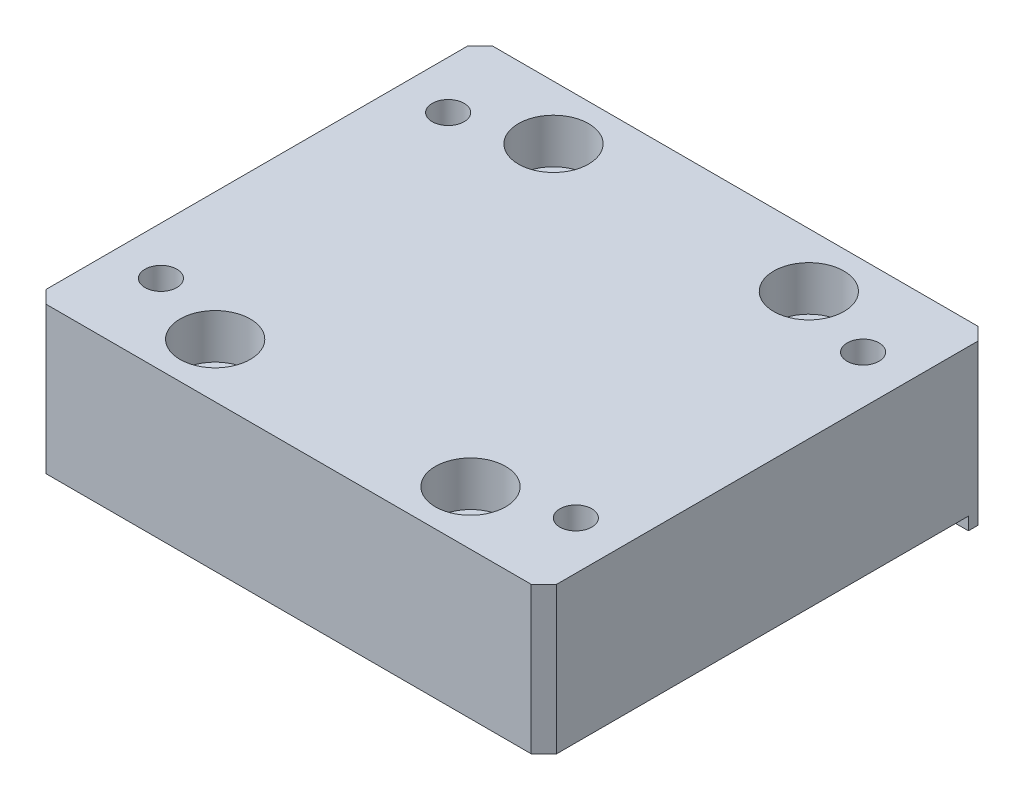
from build123d import *

# Parameters (mm, degrees)
SKETCH_1_W                = 80
SKETCH_1_H                = 70
EXTRUDE_1_DEPTH           = 12.5
SKETCH_3_W                = 80
SKETCH_3_H                = 66.5
CUT_EXTRUDE_1_DEPTH       = 2
HOLE_WIZARD_M5_1_D        = 4.2
HOLE_WIZARD_M6_1_D        = 5
CHAMFER_1_SIZE            = 2
HOLE_WIZARD_1_D           = 6.6
HOLE_WIZARD_1_DEPTH       = 25
HOLE_WIZARD_1_CBORE_D     = 11
HOLE_WIZARD_1_CBORE_DEPTH = 7


with BuildPart() as part:
    # 草图1 → 凸台-拉伸1 (new, symmetric)
    with BuildSketch(Plane(origin=(0, 0, 0), x_dir=(1, 0, 0), z_dir=(0, 1, 0))):
        Rectangle(SKETCH_1_W, SKETCH_1_H)
    extrude(amount=EXTRUDE_1_DEPTH, both=True)

    # 草图3 → 切除-拉伸1 (cut)
    with BuildSketch(Plane.XZ.offset(12.5)):
        with Locations((0, 1.75)):
            Rectangle(SKETCH_3_W, SKETCH_3_H)
    extrude(amount=-CUT_EXTRUDE_1_DEPTH, mode=Mode.SUBTRACT)

    # M5 螺纹孔1 (through all)
    with Locations(Plane(origin=(0, -10.5, 0), x_dir=(-1, 0, 0), z_dir=(0, -1, 0))):
        with Locations((20, 26.5), (-20, 26.5), (-20, -26.5), (20, -26.5)):
            Hole(HOLE_WIZARD_M5_1_D / 2)

    # M6 螺纹孔1 (through all)
    with Locations(Plane(origin=(0, -10.5, 0), x_dir=(-1, 0, 0), z_dir=(0, -1, 0))):
        with Locations((32.5, 22.5), (32.5, -22.5), (-32.5, 22.5), (-32.5, -22.5)):
            Hole(HOLE_WIZARD_M6_1_D / 2)

    # 倒角1
    chamfer_1_edges = [part.edges().sort_by_distance(p)[0] for p in [
        (-40, 0, -35),
        (40, 0, -35),
        (40, 1, 35),
        (-40, 1, 35),
    ]]
    chamfer(chamfer_1_edges, length=CHAMFER_1_SIZE)

    # 打孔尺寸(%根据)内六角花形圆柱头螺钉1
    with Locations(Plane(origin=(0, 12.5, 0), x_dir=(1, 0, 0), z_dir=(0, 1, 0))):
        with Locations((20, 26.5), (20, -26.5), (-20, -26.5), (-20, 26.5)):
            CounterBoreHole(HOLE_WIZARD_1_D / 2, HOLE_WIZARD_1_CBORE_D / 2, HOLE_WIZARD_1_CBORE_DEPTH, depth=HOLE_WIZARD_1_DEPTH)


solid = part.part
